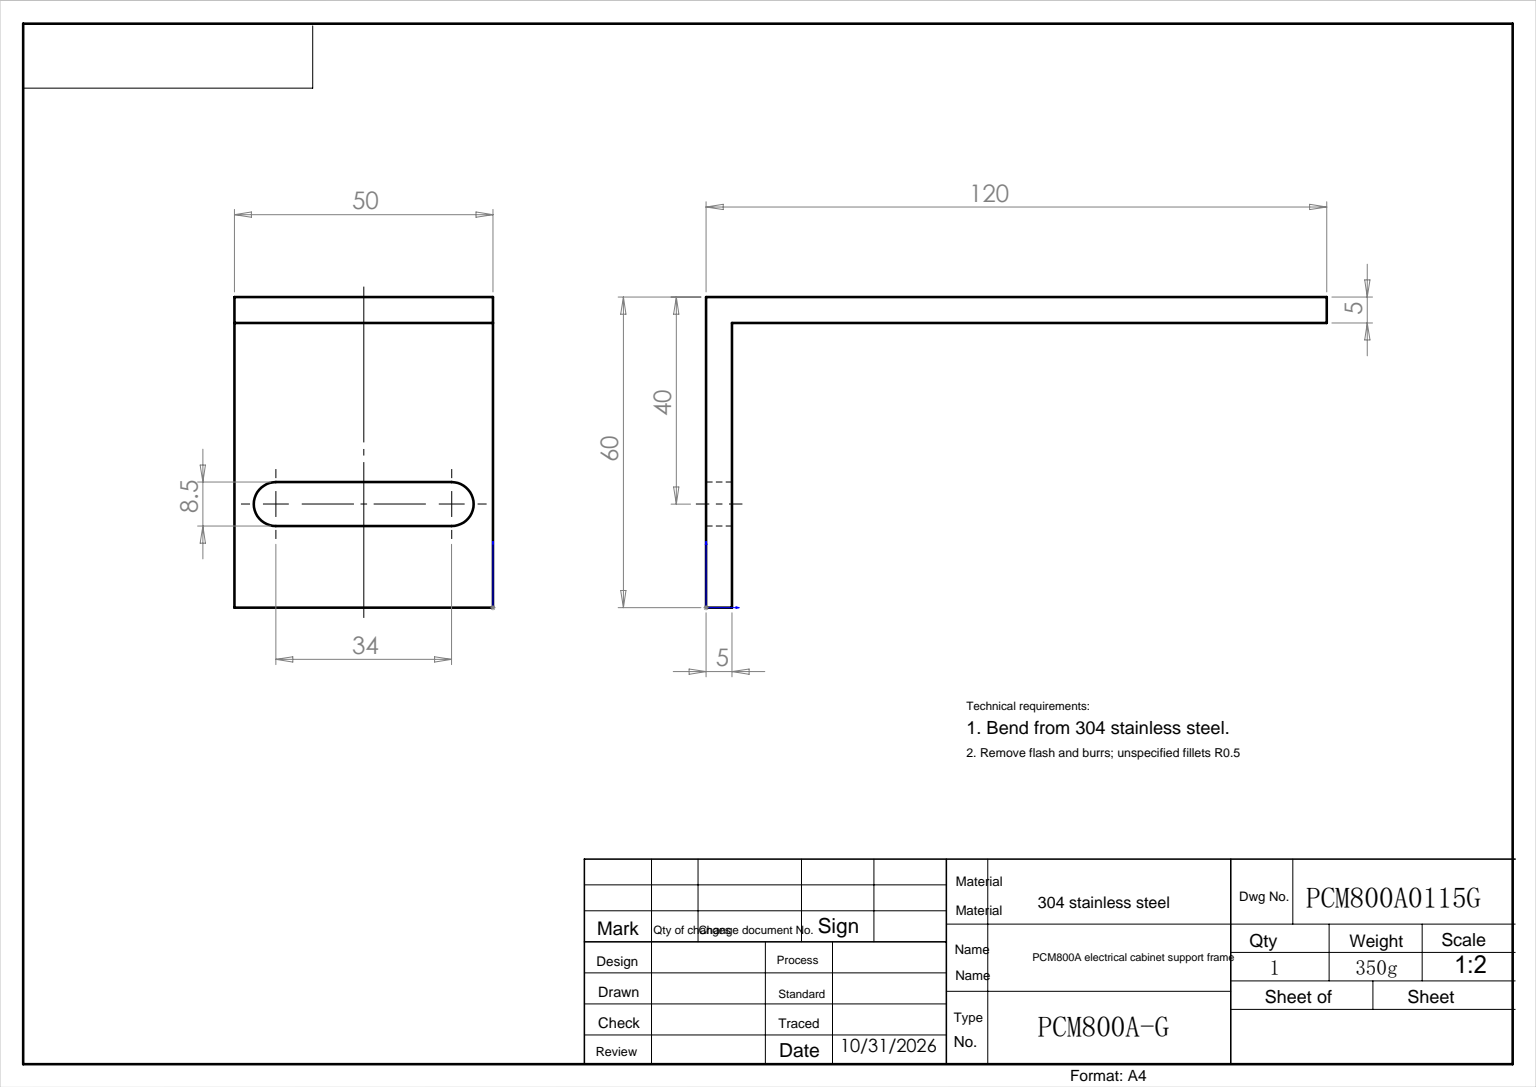
SolidWorks part; units mm, degrees
ref_plane "前视基准面" through (0, 0, 0) normal (0, 0, 1) x (1, 0, 0)
ref_plane "上视基准面" through (0, 0, 0) normal (0, 1, 0) x (1, 0, 0)
ref_plane "右视基准面" through (0, 0, 0) normal (1, 0, 0) x (0, 0, -1)
sketch "草图1" plane through (0, 0, 0) normal (0, 0, 1) x (1, 0, 0)
  line L0 (0, 0) -> (0, 60)
  line L1 (0, 60) -> (120, 60)
  dimension "D1" = 60
  dimension "D2" = 120
extrude "拉伸-薄壁1" add sketch "草图1" along normal blind 50 thin
sketch "草图2" plane through (0, 0, 0) normal (-1, 0, 0) x (0, 0, 1)
  line L0 (-3.4966, 20) -> (55.5024, 20) construction
  line L1 (50, 55) -> (0, 55) construction
  line L2 (25, 55) -> (25, -2.0641) construction
  line L3 (50, 0) -> (0, 0) construction
  line L4 (8, 24.25) -> (42, 24.25)
  line L5 (8, 15.75) -> (42, 15.75)
  arc A0 (8, 24.25) -> (8, 15.75) centre (8, 20) ccw
  arc A1 (42, 24.25) -> (42, 15.75) centre (42, 20) cw
  point P11 (25, 24.25)
  point P14 (25, 15.75)
  dimension "D2" = 8.5
  dimension "D3" = 17
  dimension "D1" = 20
extrude "切除-拉伸1" cut sketch "草图2" against normal blind 10
